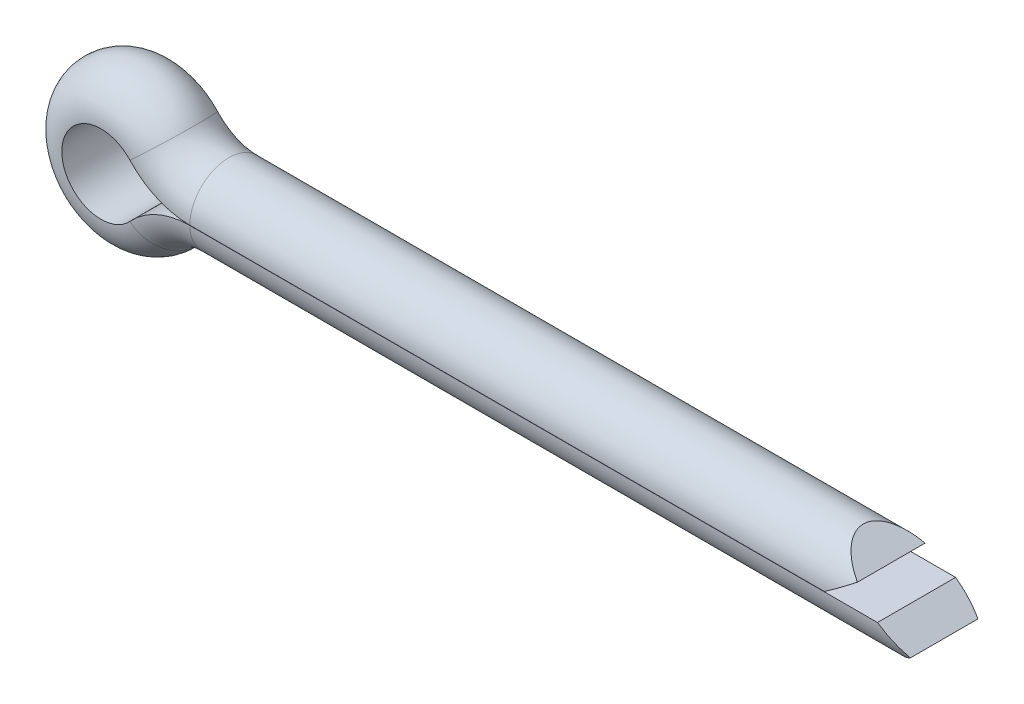
from build123d import *

# Parameters (mm, degrees)
CUT_EXTRUDE1_DEPTH      = 62.057369758
CUT_EXTRUDE1_DEPTH_BACK = 62.057369758


with BuildPart() as part:
    # Sweep2: sweep along a path in Dimension sketch
    with BuildLine(Plane.XY) as sweep2_path:
        Line((56.7, 2.95), (6.7, 2.95))
        ThreePointArc((6.7, 2.95), (5.417163248, 3.21991314), (4.351858935, 3.983883006))
        ThreePointArc((4.351858935, 3.983883006), (-5.9, 0), (4.351858935, -3.983883006))
        ThreePointArc((4.351858935, -3.983883006), (5.417163248, -3.21991314), (6.7, -2.95))
        Line((6.7, -2.95), (60.7, -2.95))
    # Sketch2 → Sweep2 (sweep)
    with BuildSketch(Plane(origin=(56.7, 2.95, 0), x_dir=(0, 0, 1), z_dir=(-1, 0, 0))):
        with BuildLine():
            Line((-2.949983051, -2.94), (2.949983051, -2.94))
            ThreePointArc((2.949983051, -2.94), (0, 0), (-2.949983051, -2.94))
        make_face()
    sweep(path=sweep2_path.line)

    # Sketch3 → Cut-Extrude1 (cut, two sides: drawn at the far end of the back side and taken through both)
    with BuildSketch(Plane.XY.offset(-CUT_EXTRUDE1_DEPTH_BACK)):
        Polygon((56.7, 1.47), (54.596982728, 2.95), (60.71, 2.95), (60.71, -2.95), (58.589980652, -2.95), (60.7, -1.48), (58.596982728, 0), (54.589980652, 0), align=None)
    extrude(amount=CUT_EXTRUDE1_DEPTH + CUT_EXTRUDE1_DEPTH_BACK, mode=Mode.SUBTRACT)


solid = part.part
